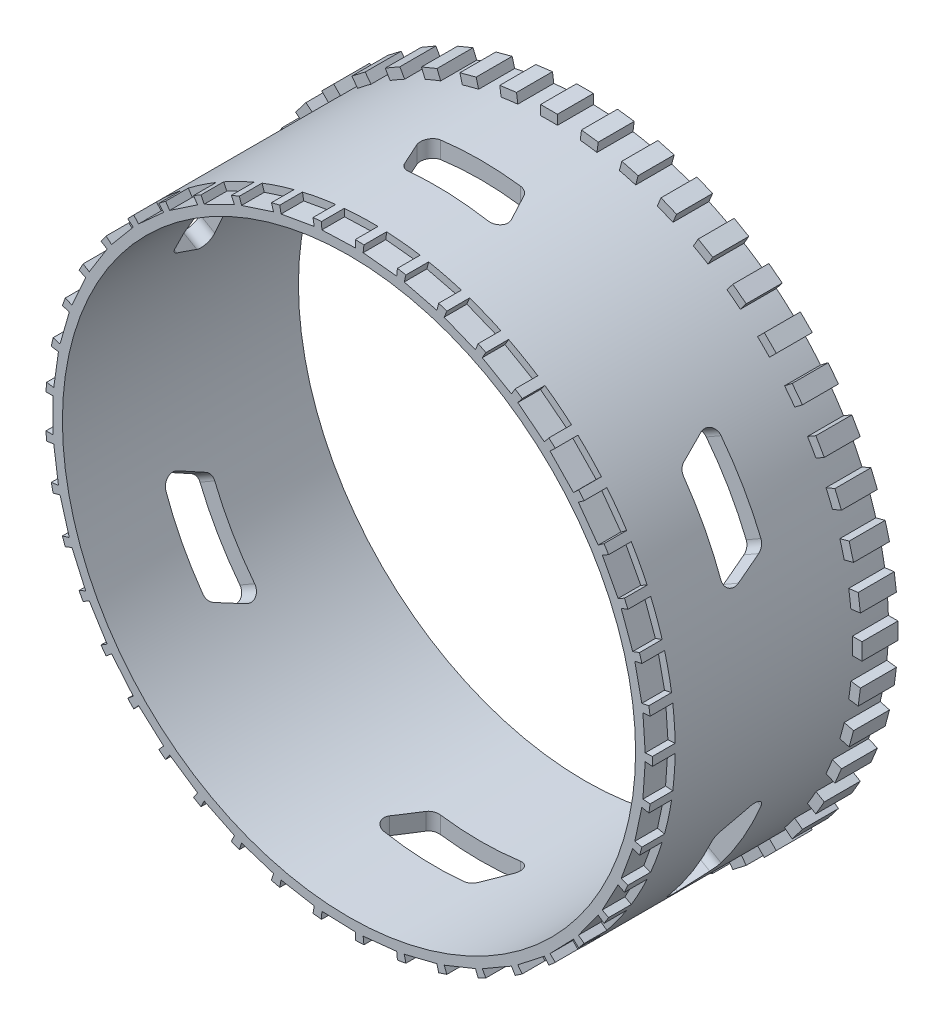
SolidWorks part; units mm, degrees
ref_plane "Front Plane" through (0, 0, 0) normal (0, 0, 1) x (1, 0, 0)
ref_plane "Top Plane" through (0, 0, 0) normal (0, 1, 0) x (1, 0, 0)
ref_plane "Right Plane" through (0, 0, 0) normal (1, 0, 0) x (0, 0, -1)
sketch "Sketch1" plane through (0, 0, 0) normal (0, 0, 1) x (1, 0, 0)
  circle A0 centre (0, 0) radius 9
  dimension "D1" = 18
extrude "Boss-Extrude1" add sketch "Sketch1" along normal blind 7
sketch "Sketch2" plane through (0, 0, 7) normal (0, 0, 1) x (1, 0, 0)
  circle A0 centre (0, 0) radius 8.5
  dimension "D1" = 17
extrude "Cut-Extrude1" cut sketch "Sketch2" against normal blind 10
sketch "Sketch6" plane through (0, 0, 0) normal (0, 1, 0) x (1, 0, 0)
  line L0 (1.1833, -3.1008) -> (-1.1833, -3.1008)
  line L1 (-1.4525, -3.2684) -> (-1.8067, -3.9884)
  line L2 (-1.5375, -4.4208) -> (0.8291, -4.4208)
  line L3 (1.0983, -4.2532) -> (1.4525, -3.5332)
  arc A0 (1.1833, -3.1008) -> (1.4525, -3.5332) centre (1.1833, -3.4008) cw
  arc A1 (1.0983, -4.2532) -> (0.8291, -4.4208) centre (0.8291, -4.1208) cw
  arc A2 (-1.5375, -4.4208) -> (-1.8067, -3.9884) centre (-1.5375, -4.1208) cw
  arc A3 (-1.4525, -3.2684) -> (-1.1833, -3.1008) centre (-1.1833, -3.4008) cw
  point P2 (0, -3.1008)
  dimension "D1" = 0.3
extrude "Cut-Extrude2" cut sketch "Sketch6" against normal blind 13
pattern_circular "CirPattern1" count 6 over 360 about axis through (0, 0, 0) along (0, 0, 1) of "Cut-Extrude2"
sketch "Sketch7" plane through (0, 0, 0) normal (0, 1, 0) x (1, 0, 0)
  line L0 (9, 0) -> (-9, 0) construction
  line L1 (-8.6437, 0) -> (-9.2824, 0)
  line L2 (-8.6437, 0) -> (-8.6437, -1.0676)
  line L3 (-8.6437, -1.0676) -> (-9.2824, -1.0676)
  line L4 (-9.2824, 0) -> (-9.2824, -1.0676)
extrude "Boss-Extrude2" add sketch "Sketch7" along normal mid plane 0.5
pattern_circular "CirPattern2" count 48 over 360 about axis through (0, 0, 0) along (0, 0, 1) of "Boss-Extrude2"
sketch "Sketch8" plane through (0, 0, 0) normal (0, 1, 0) x (1, 0, 0)
  line L1 (-9.2882, -6.3271) -> (-8.7721, -6.3271)
  line L2 (-9.2882, -6.3271) -> (-9.2882, -7.392)
  line L3 (-9.2882, -7.392) -> (-8.7721, -7.392)
  line L4 (-8.7721, -6.3271) -> (-8.7721, -7.392)
extrude "Cut-Extrude3" cut sketch "Sketch8" against normal mid plane 1
pattern_circular "CirPattern3" count 45 over 360 about axis through (0, 0, 0) along (0, 0, 1) of "Cut-Extrude3"
